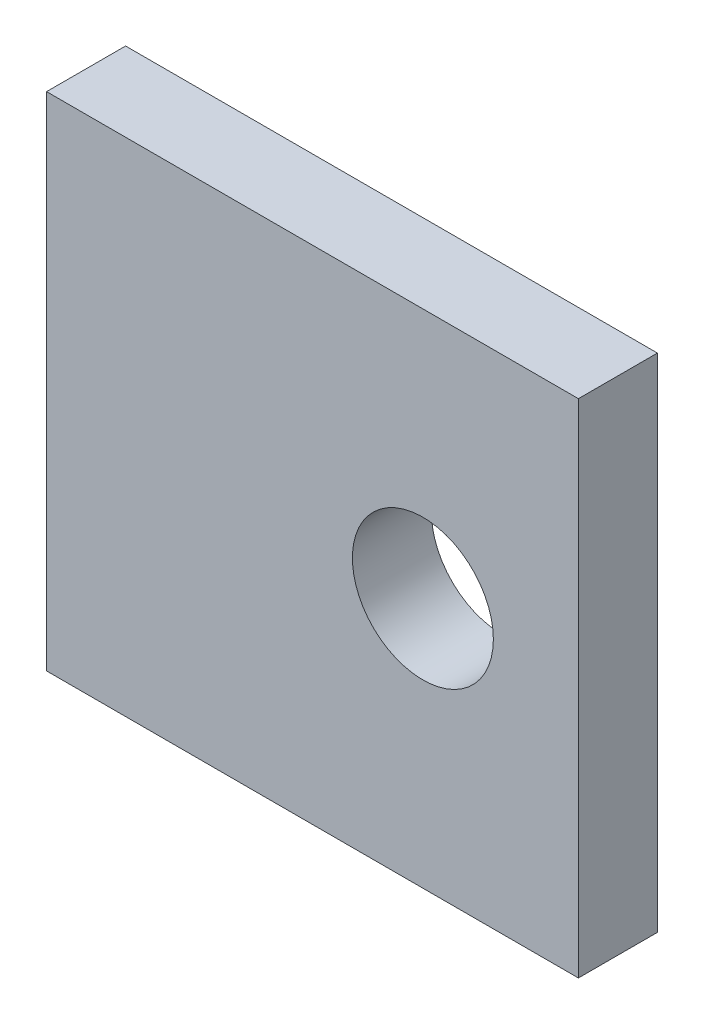
SolidWorks part; units mm, degrees
material "普通碳钢"
ref_plane "Front Plane" through (0, 0, 0) normal (0, 0, 1) x (1, 0, 0)
ref_plane "Top Plane" through (0, 0, 0) normal (0, 1, 0) x (1, 0, 0)
ref_plane "Right Plane" through (0, 0, 0) normal (1, 0, 0) x (0, 0, -1)
sketch "Sketch1" plane through (0, 0, 0) normal (0, 0, 1) x (1, 0, 0)
  line L1 (-38.1, 25.4) -> (15.748, 25.4)
  line L2 (-38.1, 25.4) -> (-38.1, -25.4)
  line L3 (-38.1, -25.4) -> (15.748, -25.4)
  line L4 (15.748, 25.4) -> (15.748, -25.4)
  circle A0 centre (0, 0) radius 7.1374
  dimension "D4" = 14.2748
  dimension "D1" = 53.848
  dimension "D2" = 50.8
  dimension "D3" = 25.4
  dimension "D5" = 15.748
extrude "Boss-Extrude1" add sketch "Sketch1" along normal mid plane 8
